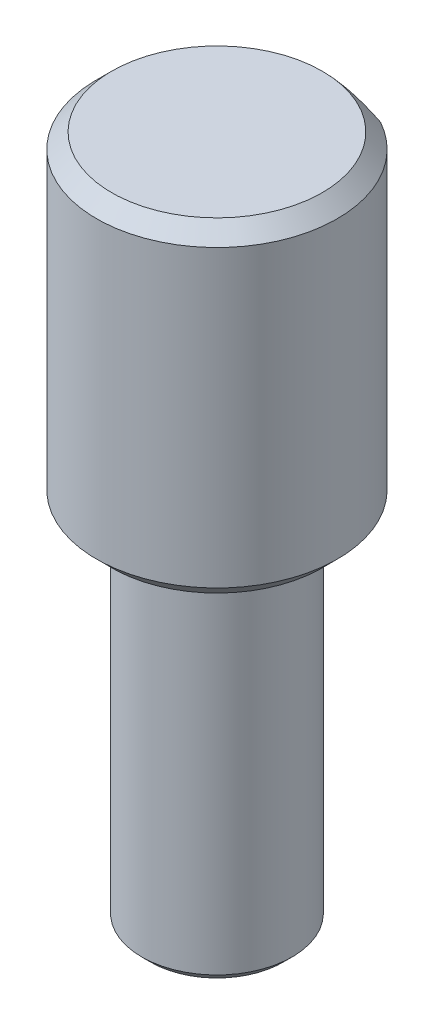
from build123d import *

# Parameters (mm, degrees)
SKETCH1_R             = 2.5
BOSS_EXTRUDE1_DEPTH   = 12
SKETCH2_R             = 4
BOSS_EXTRUDE2_DEPTH   = 10.8
CHAMFER1_SIZE         = 0.5
CHAMFER2_SIZE         = 0.3
SKETCH3_W             = 8.000389638
SKETCH3_H             = 1
CUT_EXTRUDE1_DEPTH    = 12
M3_TAPPED_HOLE1_D     = 2.5
M3_TAPPED_HOLE1_DEPTH = 7.5
M3_TAPPED_HOLE1_TIP   = 0.751075774


with BuildPart() as part:
    # Sketch1 → Boss-Extrude1 (new body)
    with BuildSketch(Plane(origin=(0, 0, 0), x_dir=(1, 0, 0), z_dir=(0, 1, 0))):
        with Locations(Location((0, 0, 0), (0, 0, 270))):
            Circle(SKETCH1_R)
    extrude(amount=BOSS_EXTRUDE1_DEPTH)

    # Sketch2 → Boss-Extrude2 (add)
    with BuildSketch(Plane(origin=(0, 12, 0), x_dir=(1, 0, 0), z_dir=(0, 1, 0))):
        with Locations(Location((0, 0, 0), (0, 0, 90))):
            Circle(SKETCH2_R)
    extrude(amount=BOSS_EXTRUDE2_DEPTH)

    # Chamfer1
    chamfer1_edges = [part.edges().sort_by_distance(p)[0] for p in [
        (0, 12, 4),
        (0, 22.8, 4),
    ]]
    chamfer(chamfer1_edges, length=CHAMFER1_SIZE)

    # Chamfer2
    chamfer2_edges = [part.edges().sort_by_distance(p)[0] for p in [
        (0, 0, -2.5),
    ]]
    chamfer(chamfer2_edges, length=CHAMFER2_SIZE)

    # Sketch3 → Cut-Extrude1 (cut)
    with BuildSketch(Plane(origin=(0, 22.8, 0), x_dir=(1, 0, 0), z_dir=(0, 1, 0))):
        with Locations((0, 4)):
            Rectangle(SKETCH3_W, SKETCH3_H)
    extrude(amount=-CUT_EXTRUDE1_DEPTH, mode=Mode.SUBTRACT)

    # M3 Tapped Hole1
    with Locations(Plane(origin=(0, 0, 0), x_dir=(-1, 0, 0), z_dir=(0, -1, 0))):
        with Locations((0, 0)):
            Hole(M3_TAPPED_HOLE1_D / 2, depth=M3_TAPPED_HOLE1_DEPTH)
            with Locations((0, 0, -(M3_TAPPED_HOLE1_DEPTH + M3_TAPPED_HOLE1_TIP / 2))):  # 118° drill point
                Cone(0, M3_TAPPED_HOLE1_D / 2, M3_TAPPED_HOLE1_TIP, mode=Mode.SUBTRACT)


solid = part.part
